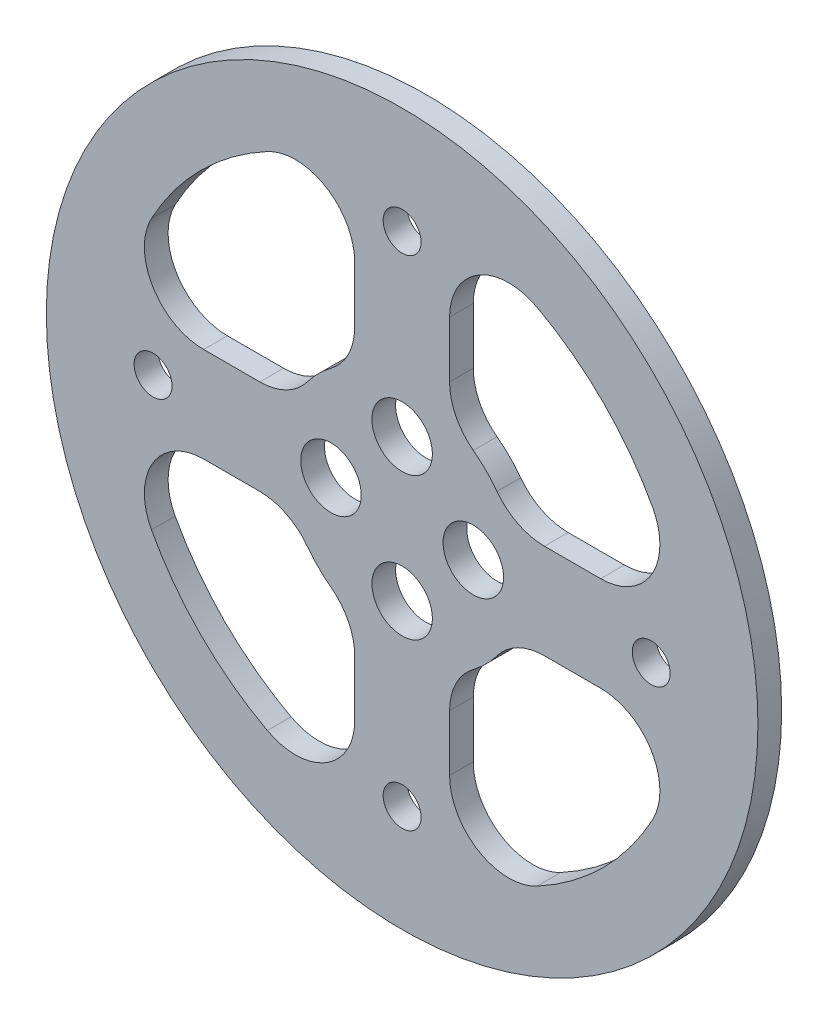
from build123d import *

# Parameters (mm, degrees)
SKETCH_1_R          = 30
EXTRUDE_1_DEPTH     = 2
SKETCH_2_R          = 1.6
CUT_EXTRUDE_1_DEPTH = 10
SKETCH_3_R          = 2.55
CUT_EXTRUDE_2_DEPTH = 10


with BuildPart() as part:
    # 草图1 → 凸台-拉伸1 (new body)
    with BuildSketch(Plane.XY):
        Circle(SKETCH_1_R)
        with BuildLine():
            Line((4, 16.733200531), (4, 12))
            ThreePointArc((4, 12), (4.527864045, 9.763932023), (6, 8))
            ThreePointArc((6, 8), (7.071067812, 7.071067812), (8, 6))
            ThreePointArc((8, 6), (9.763932023, 4.527864045), (12, 4))
            Line((12, 4), (16.733200531, 4))
            ThreePointArc((16.733200531, 4), (21.025175907, 6.43505412), (21.136674355, 11.368421053))
            ThreePointArc((21.136674355, 11.368421053), (16.970562748, 16.970562748), (11.368421053, 21.136674355))
            ThreePointArc((11.368421053, 21.136674355), (6.43505412, 21.025175907), (4, 16.733200531))
        make_face(mode=Mode.SUBTRACT)
        with BuildLine():
            Line((-4, 16.733200531), (-4, 12))
            ThreePointArc((-4, 12), (-4.527864045, 9.763932023), (-6, 8))
            ThreePointArc((-6, 8), (-7.071067812, 7.071067812), (-8, 6))
            ThreePointArc((-8, 6), (-9.763932023, 4.527864045), (-12, 4))
            Line((-12, 4), (-16.733200531, 4))
            ThreePointArc((-16.733200531, 4), (-21.025175907, 6.43505412), (-21.136674355, 11.368421053))
            ThreePointArc((-21.136674355, 11.368421053), (-16.970562748, 16.970562748), (-11.368421053, 21.136674355))
            ThreePointArc((-11.368421053, 21.136674355), (-6.43505412, 21.025175907), (-4, 16.733200531))
        make_face(mode=Mode.SUBTRACT)
        with BuildLine():
            Line((16.733200531, -4), (12, -4))
            ThreePointArc((12, -4), (9.763932023, -4.527864045), (8, -6))
            ThreePointArc((8, -6), (7.071067812, -7.071067812), (6, -8))
            ThreePointArc((6, -8), (4.527864045, -9.763932023), (4, -12))
            Line((4, -12), (4, -16.733200531))
            ThreePointArc((4, -16.733200531), (6.43505412, -21.025175907), (11.368421053, -21.136674355))
            ThreePointArc((11.368421053, -21.136674355), (16.970562748, -16.970562748), (21.136674355, -11.368421053))
            ThreePointArc((21.136674355, -11.368421053), (21.025175907, -6.43505412), (16.733200531, -4))
        make_face(mode=Mode.SUBTRACT)
        with BuildLine():
            Line((-4, -16.733200531), (-4, -12))
            ThreePointArc((-4, -12), (-4.527864045, -9.763932023), (-6, -8))
            ThreePointArc((-6, -8), (-7.071067812, -7.071067812), (-8, -6))
            ThreePointArc((-8, -6), (-9.763932023, -4.527864045), (-12, -4))
            Line((-12, -4), (-16.733200531, -4))
            ThreePointArc((-16.733200531, -4), (-21.025175907, -6.43505412), (-21.136674355, -11.368421053))
            ThreePointArc((-21.136674355, -11.368421053), (-16.970562748, -16.970562748), (-11.368421053, -21.136674355))
            ThreePointArc((-11.368421053, -21.136674355), (-6.43505412, -21.025175907), (-4, -16.733200531))
        make_face(mode=Mode.SUBTRACT)
    extrude(amount=EXTRUDE_1_DEPTH)

    # 草图2 → 切除-拉伸1 (cut)
    with BuildSketch(Plane.XY.offset(2)):
        with Locations((-21, 0)):
            Circle(SKETCH_2_R)
        with Locations((0, 21)):
            Circle(SKETCH_2_R)
        with Locations((21, 0)):
            Circle(SKETCH_2_R)
        with Locations((0, -21)):
            Circle(SKETCH_2_R)
    extrude(amount=-CUT_EXTRUDE_1_DEPTH, mode=Mode.SUBTRACT)

    # 草图3 → 切除-拉伸2 (cut)
    with BuildSketch(Plane.XY.offset(2)):
        with Locations((0, 6)):
            Circle(SKETCH_3_R)
        with Locations((-6, 0)):
            Circle(SKETCH_3_R)
        with Locations((6, 0)):
            Circle(SKETCH_3_R)
        with Locations((0, -6)):
            Circle(SKETCH_3_R)
    extrude(amount=-CUT_EXTRUDE_2_DEPTH, mode=Mode.SUBTRACT)


solid = part.part
